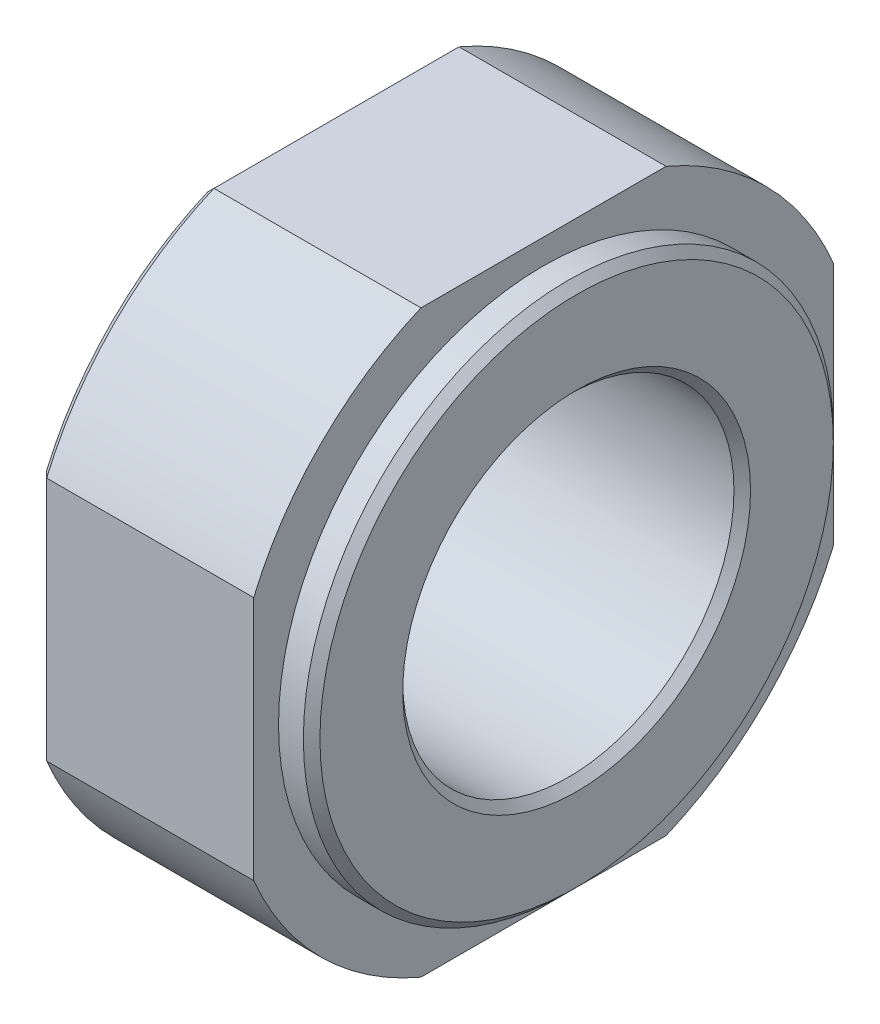
from build123d import *

# Parameters (mm, degrees)
SKETCH1_R           = 19
SKETCH1_R_2         = 10
BOSS_EXTRUDE1_DEPTH = 15
SKETCH2_OUTSIDE_W   = 51.158
SKETCH2_OUTSIDE_H   = 51.158
SKETCH2_OUTSIDE_R   = 16
CUT_EXTRUDE1_DEPTH  = 2
SKETCH3_OUTSIDE_W   = 51.158
SKETCH3_OUTSIDE_H   = 51.158
SKETCH3_OUTSIDE_W_2 = 35
SKETCH3_OUTSIDE_H_2 = 35
CUT_EXTRUDE2_DEPTH  = 31.773365107
CHAMFER1_SIZE       = 0.5


with BuildPart() as part:
    # Sketch1 → Boss-Extrude1 (new body)
    with BuildSketch(Plane(origin=(0, 0, 0), x_dir=(0, 0, -1), z_dir=(1, 0, 0))):
        Circle(SKETCH1_R)
        Circle(SKETCH1_R_2, mode=Mode.SUBTRACT)
    extrude(amount=BOSS_EXTRUDE1_DEPTH)

    # Sketch2 outside → Cut-Extrude1 (cut)
    with BuildSketch(Plane(origin=(15, 0, 0), x_dir=(0, 0, -1), z_dir=(1, 0, 0))):
        Rectangle(SKETCH2_OUTSIDE_W, SKETCH2_OUTSIDE_H)
        Circle(SKETCH2_OUTSIDE_R, mode=Mode.SUBTRACT)
    extrude(amount=-CUT_EXTRUDE1_DEPTH, mode=Mode.SUBTRACT)

    # Sketch3 outside → Cut-Extrude2 (cut, through all)
    with BuildSketch(Plane.ZY):
        Rectangle(SKETCH3_OUTSIDE_W, SKETCH3_OUTSIDE_H)
        Rectangle(SKETCH3_OUTSIDE_W_2, SKETCH3_OUTSIDE_H_2, mode=Mode.SUBTRACT)
    extrude(amount=-CUT_EXTRUDE2_DEPTH, mode=Mode.SUBTRACT)

    # Chamfer1
    chamfer1_edges = [part.edges().sort_by_distance(p)[0] for p in [
        (15, 0, 16),
        (0, 13.435028843, -13.435028843),
        (0, 13.435028843, 13.435028843),
        (0, -13.435028843, 13.435028843),
        (0, -13.435028843, -13.435028843),
        (0, 0, 17.5),
        (0, -17.5, 0),
        (0, 0, -17.5),
        (0, 17.5, 0),
        (0, 0, 10),
        (15, 0, 10),
    ]]
    chamfer(chamfer1_edges, length=CHAMFER1_SIZE)


solid = part.part
